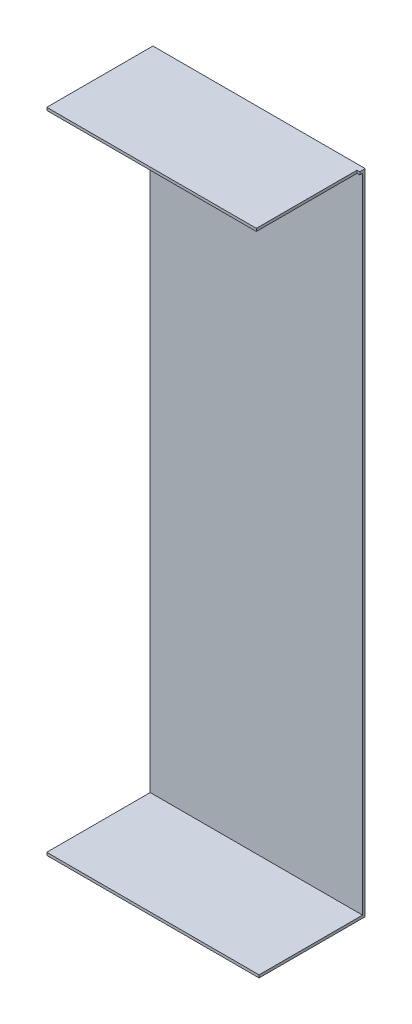
from build123d import *

# Parameters (mm, degrees)
SKETCH1_W           = 77
SKETCH1_H           = 238
BOSS_EXTRUDE1_DEPTH = 1
SKETCH2_W           = 77
SKETCH2_H           = 1
BOSS_EXTRUDE2_DEPTH = 38
BOSS_EXTRUDE3_DEPTH = 1


with BuildPart() as part:
    # Sketch1 → Boss-Extrude1 (new body)
    with BuildSketch(Plane.XY):
        Rectangle(SKETCH1_W, SKETCH1_H)
    extrude(amount=BOSS_EXTRUDE1_DEPTH)

    # Sketch2 → Boss-Extrude2 (add)
    with BuildSketch(Plane.XY.offset(1)):
        with Locations((0, 118.5)):
            Rectangle(SKETCH2_W, SKETCH2_H)
        with Locations((0, -118.5)):
            Rectangle(SKETCH2_W, SKETCH2_H)
    extrude(amount=BOSS_EXTRUDE2_DEPTH)

    # Sketch3 → Boss-Extrude3 (add)
    with BuildSketch(Plane(origin=(38.5, 0, 0), x_dir=(0, 0, -1), z_dir=(1, 0, 0))):
        Polygon((-2, 119), (-2, 118), (-1, 118), (-1, -118), (-39, -118), (-39, -119), (0, -119), (0, 119), align=None)
    extrude(amount=BOSS_EXTRUDE3_DEPTH)


solid = part.part
